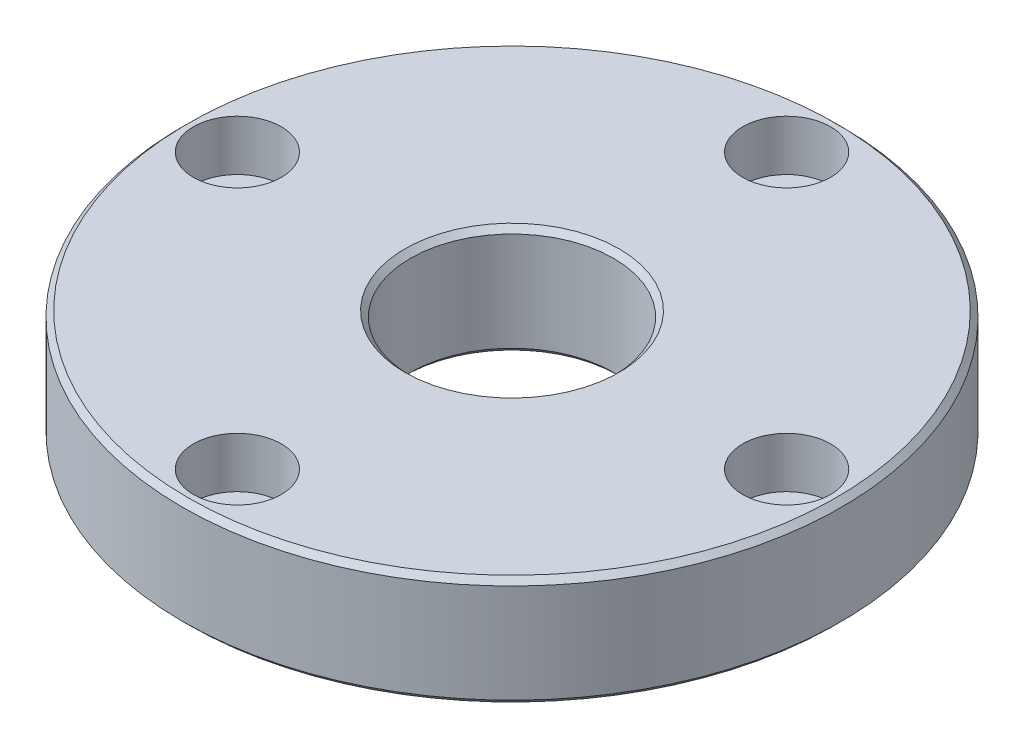
SolidWorks part; units mm, degrees
ref_plane "前视基准面" through (0, 0, 0) normal (0, 0, 1) x (1, 0, 0)
ref_plane "上视基准面" through (0, 0, 0) normal (0, 1, 0) x (1, 0, 0)
ref_plane "右视基准面" through (0, 0, 0) normal (1, 0, 0) x (0, 0, -1)
sketch "草图1" plane through (0, 0, 0) normal (0, 1, 0) x (1, 0, 0)
  circle A0 centre (0, 0) radius 30
  dimension "D1" = 60
extrude "凸台-拉伸1" add sketch "草图1" along normal blind 10
hole_wizard "M20x1.5 螺纹孔1" positions "草图3" profile "草图2" tap size "M20x1.5" standard "GB" end condition through all
sketch "草图3" plane through (0, 10, 0) normal (0, 1, 0) x (1, 0, 0)
  point P0 (0, 0)
sketch "草图2" plane through (0, 10, 0) normal (1, 0, 0) x (0, 0, 1)
  line L0 (0, 0) -> (0, 10)
  line L1 (0, 10) -> (9.25, 10)
  line L2 (9.25, 10) -> (9.25, 0)
  line L5 (9.25, 0) -> (0, 0)
  line L11 (0, -6.35) -> (0, 107.95) construction
  dimension "通孔螺纹孔钻头直径" = 18.5
  dimension "通孔螺纹孔钻头深度" = 10
cosmetic thread "孔螺蚊线1"
hole_wizard "打孔尺寸(%根据)内六角圆柱头螺钉的类型1" positions "草图5" profile "草图4" counterbore size "M4" standard "GB" end condition through all
sketch "草图5" plane through (0, 10, 0) normal (0, 1, 0) x (1, 0, 0)
  point P0 (0, 25)
  point P8 (25, 0)
  point P9 (0, -25)
  point P10 (-25, 0)
  dimension "D1" = 25
sketch "草图4" plane through (0, 10, -25) normal (1, 0, 0) x (0, 0, 1)
  line L0 (0, 0) -> (0, 10)
  line L1 (0, 10) -> (2.25, 10)
  line L3 (2.25, 10) -> (2.25, 4.6)
  line L4 (2.25, 4.6) -> (4, 4.6)
  line L5 (4, 4.6) -> (4, 0)
  line L7 (4, 0) -> (0, 0)
  line L11 (0, -6.35) -> (0, 107.95) construction
  dimension "通孔孔直径" = 4.5
  dimension "通孔孔深度" = 10
  dimension "柱形沉头孔直径" = 8
  dimension "柱形沉头孔深度" = 4.6
chamfer "倒角1" distance 0.5 angle 45 4 edges at (0, 0, 30) (0, 10, 30) (0, 0, 9.25) (0, 10, 9.25)
